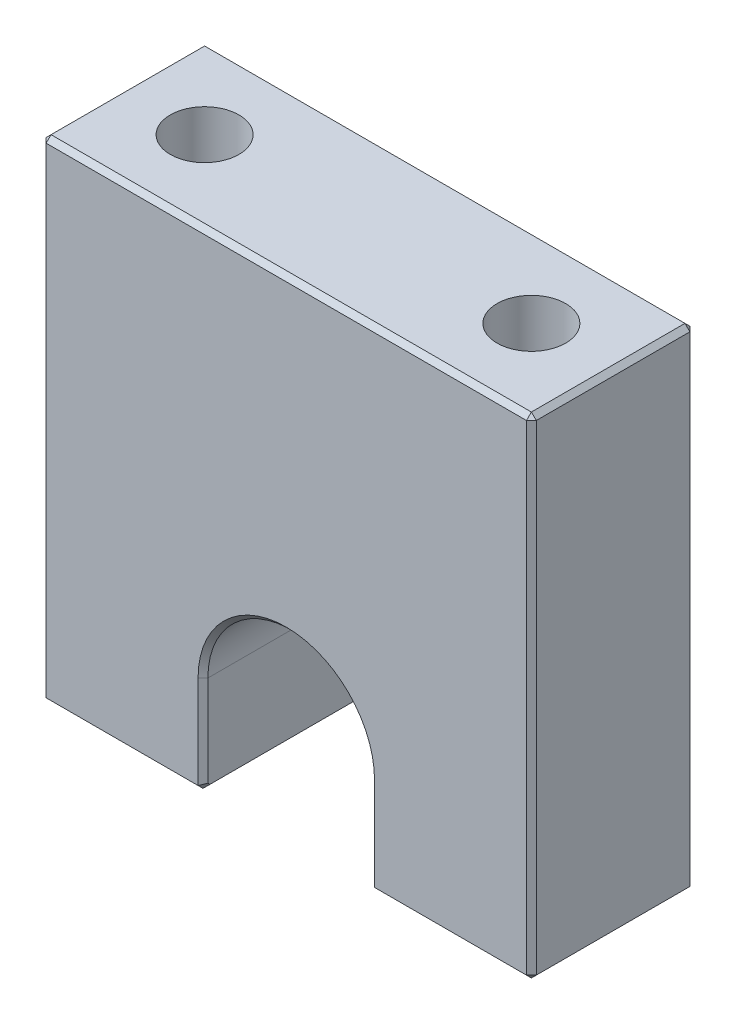
SolidWorks part; units mm, degrees
material "Al6061"
ref_plane "Front" through (0, 0, 0) normal (0, 0, 1) x (1, 0, 0)
ref_plane "Top" through (0, 0, 0) normal (0, 1, 0) x (1, 0, 0)
ref_plane "Right" through (0, 0, 0) normal (1, 0, 0) x (0, 0, -1)
sketch "草图1" plane through (0, 0, 0) normal (0, 0, 1) x (1, 0, 0)
  line L1 (-15, 15) -> (15, 15)
  line L2 (-15, 15) -> (-15, -15)
  line L3 (-15, -15) -> (15, -15)
  line L4 (15, 15) -> (15, -15)
  line L5 (-15, 15) -> (15, -15) construction
  line L6 (-15, -15) -> (15, 15) construction
  point P0 (0, 0)
  dimension "D1" = 30
  dimension "D2" = 30
extrude "凸台-拉伸1" add sketch "草图1" along normal blind 10
hole_wizard "M5 螺纹孔1" positions "草图3" profile "草图2" tap size "M5" standard "Iso"
sketch "草图3" plane through (9.1012, 15, -0.3606) normal (0, -1, 0) x (-1, 0, 0)
  line L0 (9.1012, -0.3606) -> (9.1012, -10.3606) construction
  line L1 (24.1012, -10.3606) -> (-5.8988, -10.3606) construction
  line L3 (24.1012, -5.3606) -> (19.1012, -5.3606) construction
  line L4 (24.1012, -10.3606) -> (24.1012, -0.3606) construction
  point P0 (-0.8988, -5.3606)
  point P2 (19.1012, -5.3606)
  dimension "D1" = 20
sketch "草图2" plane through (10, 15, 5) normal (1, 0, 0) x (0, 0, 1)
  line L0 (0, 0) -> (0, 17.2618)
  line L1 (0, 17.2618) -> (2.1, 16)
  line L2 (2.1, 16) -> (2.1, 0)
  line L5 (2.1, 0) -> (0, 0)
  line L10 (0, 17.2618) -> (-2.1, 16) construction
  line L11 (0, -6.35) -> (0, 107.95) construction
  dimension "螺纹孔钻头直径" = 4.2
  dimension "螺纹孔钻头深度" = 16
  dimension "导头角度" = 118
cosmetic thread "孔螺蚊线1" parameters "D1"=12, "D2"=5
cosmetic thread "孔螺蚊线2" parameters "D1"=12, "D2"=5
chamfer "倒角1" distance 0.3 angle 45 12 edges at (0, 15, 10) (0, 15, 0) (15, -15, 5) (15, 0, 10) (15, 15, 5) (15, 0, 0) (-15, 15, 5) (-15, 0, 10) (-15, 0, 0) (0, -15, 0) (-15, -15, 5) (0, -15, 10)
sketch "草图4" plane through (0, 0, 10) normal (0, 0, 1) x (1, 0, 0)
  line L0 (0, -15) -> (0, -9) construction
  line L1 (14.7, -15) -> (-14.7, -15) construction
  line L2 (-5.1, -15) -> (-5.1, -9)
  line L3 (5.1, -15) -> (5.1, -9)
  arc A0 (-5.1, -15) -> (5.1, -15) centre (0, -15) ccw
  arc A1 (5.1, -9) -> (-5.1, -9) centre (0, -9) ccw
  point P5 (0, -12)
  dimension "D2" = 5.1
  dimension "D1" = 6
extrude "切除-拉伸1" cut sketch "草图4" against normal through all
chamfer "倒角2" distance 0.3 angle 45 12 edges at (5.1, -14.85, 9.85) (5.1, -14.85, 0.15) (5.1, -15, 5) (-5.1, -14.85, 0.15) (-5.1, -14.85, 9.85) (-5.1, -15, 5) (5.1, -11.85, 0) (-5.1, -11.85, 0) (0, -3.9, 0) (5.1, -11.85, 10) (-5.1, -11.85, 10) (0, -3.9, 10)
